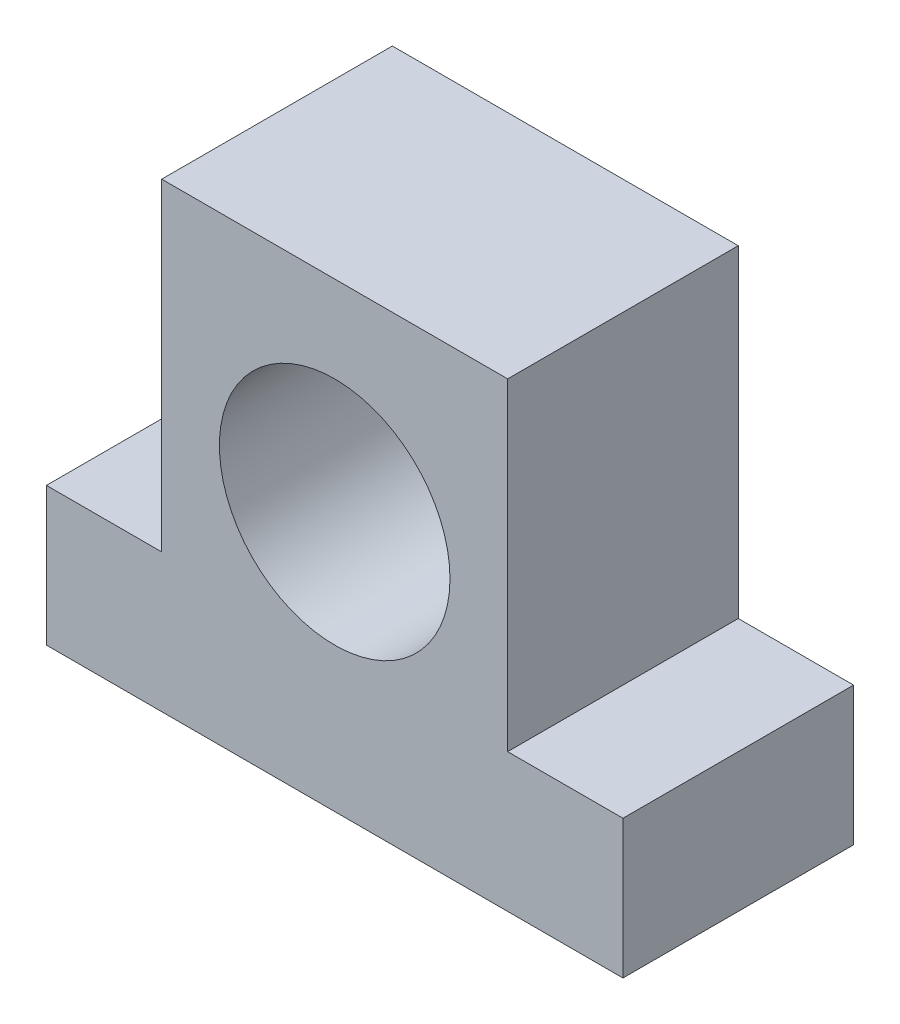
SolidWorks part; units mm, degrees
ref_plane "前视基准面" through (0, 0, 0) normal (0, 0, 1) x (1, 0, 0)
ref_plane "上视基准面" through (0, 0, 0) normal (0, 1, 0) x (1, 0, 0)
ref_plane "右视基准面" through (0, 0, 0) normal (1, 0, 0) x (0, 0, -1)
sketch "草图1" plane through (0, 0, 0) normal (0, 0, 1) x (1, 0, 0)
  line L1 (-25, -20) -> (25, -20)
  line L2 (-25, -20) -> (-25, 20)
  line L3 (-25, 20) -> (25, 20)
  line L4 (25, -20) -> (25, 20)
  line L5 (-25, -20) -> (25, 20) construction
  line L6 (-25, 20) -> (25, -20) construction
  point P0 (0, 0)
  dimension "D1" = 50
  dimension "D2" = 40
extrude "凸台-拉伸1" add sketch "草图1" along normal blind 20
sketch "草图2" plane through (0, 0, 20) normal (0, 0, 1) x (1, 0, 0)
  line L0 (0, 0) -> (0, 20) construction
  line L1 (25, 20) -> (-25, 20) construction
  line L2 (-25, -20) -> (25, -20) construction
  circle A0 centre (0, 2.5) radius 10
  dimension "D1" = 20
  dimension "D2" = 22.5
extrude "切除-拉伸1" cut sketch "草图2" against normal through all
sketch "草图3" plane through (0, 0, 20) normal (0, 0, 1) x (1, 0, 0)
  line L0 (0, 0) -> (0, 20) construction
  line L1 (-25, 20) -> (-15, 20)
  line L2 (-25, 20) -> (-25, -8)
  line L3 (-25, -8) -> (-15, -8)
  line L4 (-15, 20) -> (-15, -8)
  line L5 (25, 20) -> (15, 20)
  line L6 (25, 20) -> (25, -8)
  line L7 (25, -8) -> (15, -8)
  line L8 (15, 20) -> (15, -8)
  line L9 (25, 20) -> (-25, 20) construction
  line L10 (-25, -20) -> (25, -20) construction
  dimension "D1" = 10
  dimension "D2" = 12
extrude "切除-拉伸2" cut sketch "草图3" against normal through all
